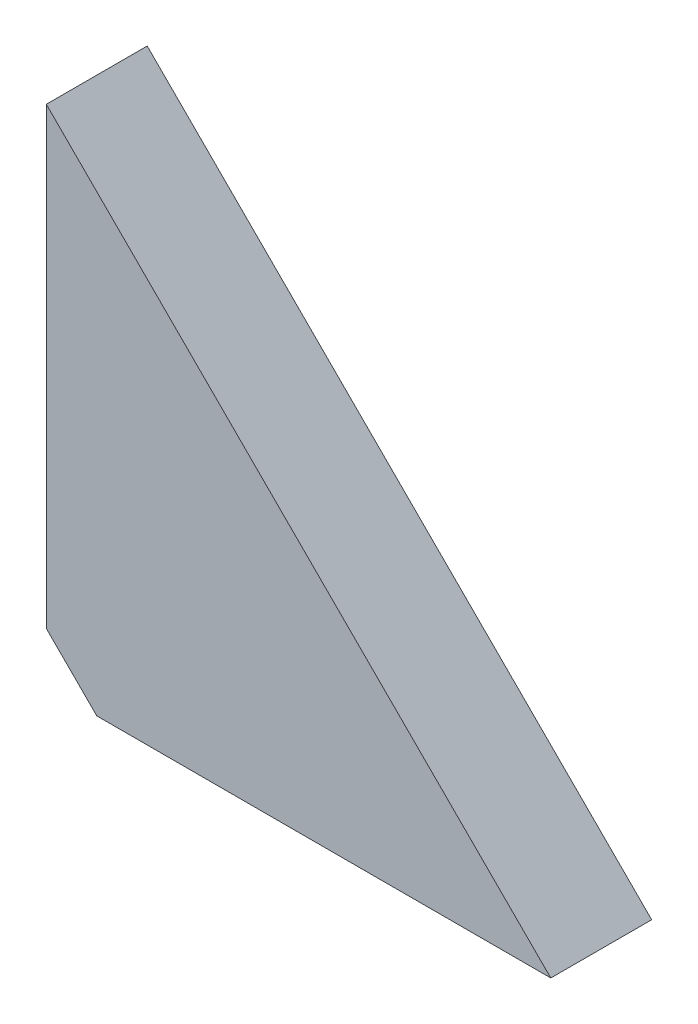
SolidWorks part; units mm, degrees
material "Q235B"
ref_plane "Front Plane" through (0, 0, 0) normal (0, 0, 1) x (1, 0, 0)
ref_plane "Top Plane" through (0, 0, 0) normal (0, 1, 0) x (1, 0, 0)
ref_plane "Right Plane" through (0, 0, 0) normal (1, 0, 0) x (0, 0, -1)
sketch "Sketch1" plane through (0, 0, 0) normal (0, 0, 1) x (1, 0, 0)
  line L0 (0, 0) -> (0, 50)
  line L1 (0, 50) -> (50, 0)
  line L2 (50, 0) -> (0, 0)
  dimension "D1" = 50
  dimension "D2" = 50
extrude "Boss-Extrude1" add sketch "Sketch1" along normal mid plane 10
chamfer "Chamfer1" distance 5 angle 45 1 edges at (0, 0, 0)
